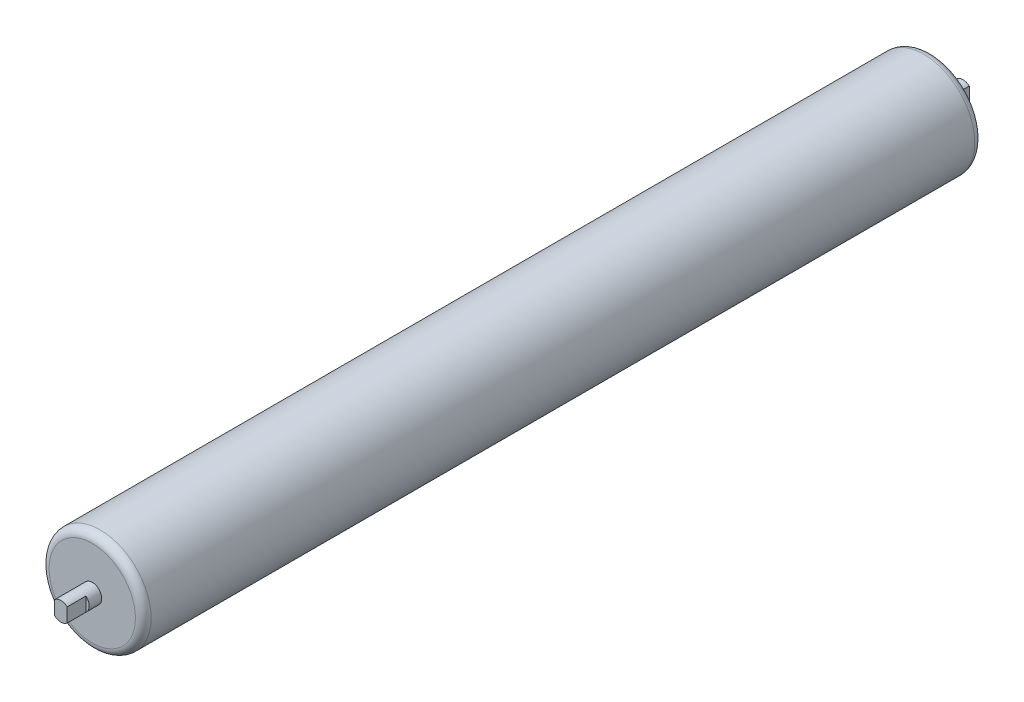
from build123d import *

# Parameters (mm, degrees)
SKETCH_1_R           = 32.5
EXTRUDE_1_DEPTH      = 267.5
SKETCH_2_R           = 6
EXTRUDE_2_DEPTH      = 20
SKETCH_3_OUTSIDE_W   = 179.512
SKETCH_3_OUTSIDE_H   = 179.512
SKETCH_3_OUTSIDE_W_2 = 8
SKETCH_3_OUTSIDE_H_2 = 12.842917612
CUT_EXTRUDE_1_DEPTH  = 12
FILLET_1_R           = 5


with BuildPart() as part:
    # 草图1 → 凸台-拉伸1 (new, symmetric)
    with BuildSketch(Plane.XY):
        Circle(SKETCH_1_R)
    extrude(amount=EXTRUDE_1_DEPTH, both=True)

    # 草图2 → 凸台-拉伸2 (add)
    with BuildSketch(Plane(origin=(0, 0, -267.5), x_dir=(-1, 0, 0), z_dir=(0, 0, -1))):
        with Locations(Location((0, 0, 0), (0, 0, 180))):
            Circle(SKETCH_2_R)
    extrude_2 = extrude(amount=EXTRUDE_2_DEPTH)

    # 草图3 outside → 切除-拉伸1 (cut)
    with BuildSketch(Plane(origin=(0, 0, -287.5), x_dir=(-1, 0, 0), z_dir=(0, 0, -1))):
        Rectangle(SKETCH_3_OUTSIDE_W, SKETCH_3_OUTSIDE_H)
        Rectangle(SKETCH_3_OUTSIDE_W_2, SKETCH_3_OUTSIDE_H_2, mode=Mode.SUBTRACT)
    cut_extrude_1 = extrude(amount=-CUT_EXTRUDE_1_DEPTH, mode=Mode.SUBTRACT)

    # 镜向1: 凸台-拉伸2, 切除-拉伸1 across plane
    add(extrude_2.mirror(Plane.XY))
    add(cut_extrude_1.mirror(Plane.XY), mode=Mode.SUBTRACT)

    # 圆角1
    fillet_1_edges = [part.edges().sort_by_distance(p)[0] for p in [
        (-32.5, 0, -267.5),
        (-32.5, 0, 267.5),
    ]]
    fillet(fillet_1_edges, radius=FILLET_1_R)


solid = part.part
